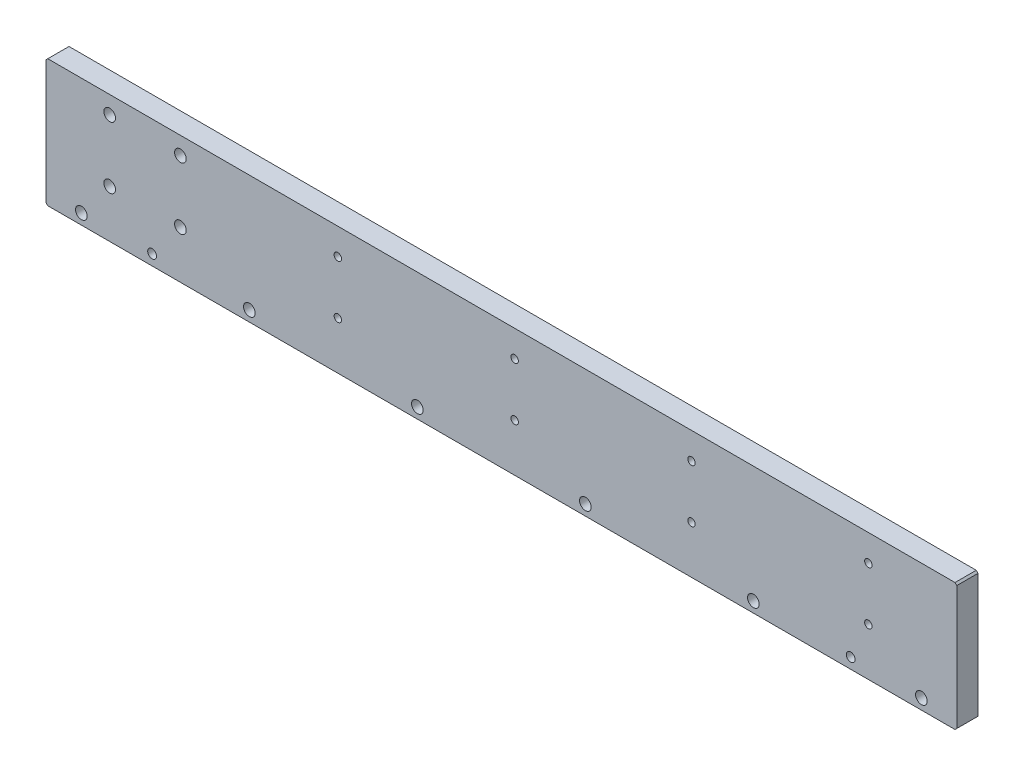
from build123d import *

# Parameters (mm, degrees)
SKETCH1_W                                           = 515
SKETCH1_H                                           = 72
BOSS_EXTRUDE1_DEPTH                                 = 6
M5_TAPPED_HOLE1_D                                   = 4.2
BLIND_PIN_HOLE0_D                                   = 5
BLIND_PIN_HOLE0_DEPTH                               = 10
BLIND_PIN_HOLE0_TIP                                 = 1.502151548
CBORE_FOR_M6_HEX_SOCKET_HEAD_CAP_SCREW1_D           = 6.6
CBORE_FOR_M6_HEX_SOCKET_HEAD_CAP_SCREW1_CBORE_D     = 11
CBORE_FOR_M6_HEX_SOCKET_HEAD_CAP_SCREW1_CBORE_DEPTH = 6.4
BLIND_PIN_HOLE1_D                                   = 5
BLIND_PIN_HOLE1_DEPTH                               = 10
BLIND_PIN_HOLE1_TIP                                 = 1.502151548
CBORE_FOR_M6_HEX_SOCKET_HEAD_CAP_SCREW2_D           = 6.6
CBORE_FOR_M6_HEX_SOCKET_HEAD_CAP_SCREW2_CBORE_D     = 11
CBORE_FOR_M6_HEX_SOCKET_HEAD_CAP_SCREW2_CBORE_DEPTH = 6.4
CHAMFER1_SIZE                                       = 1


with BuildPart() as part:
    # Sketch1 → Boss-Extrude1 (new, symmetric)
    with BuildSketch(Plane.XY):
        Rectangle(SKETCH1_W, SKETCH1_H)
    extrude(amount=BOSS_EXTRUDE1_DEPTH, both=True)

    # M5 Tapped Hole1 (through all)
    with Locations(Plane.XY.offset(6)):
        with Locations((207.5, -9), (207.5, 21), (107.5, -9), (107.5, 21), (7.5, -9), (7.5, 21), (-92.5, -9), (-92.5, 21)):
            Hole(M5_TAPPED_HOLE1_D / 2)

    # Blind pin hole0
    with Locations(Plane(origin=(0, 0, -6), x_dir=(1, 0, 0), z_dir=(0, 0, -1))):
        with Locations((227.5, 26.5), (-122.5, 26.5)):
            Hole(BLIND_PIN_HOLE0_D / 2, depth=BLIND_PIN_HOLE0_DEPTH)
            with Locations((0, 0, -(BLIND_PIN_HOLE0_DEPTH + BLIND_PIN_HOLE0_TIP / 2))):  # 118° drill point
                Cone(0, BLIND_PIN_HOLE0_D / 2, BLIND_PIN_HOLE0_TIP, mode=Mode.SUBTRACT)

    # CBORE for M6 Hex Socket Head Cap Screw1 (through all)
    with Locations(Plane(origin=(0, 0, -6), x_dir=(1, 0, 0), z_dir=(0, 0, -1))):
        with Locations((-237.5, 30), (-142.5, 30), (-47.5, 30), (47.5, 30), (142.5, 30), (237.5, 30)):
            CounterBoreHole(CBORE_FOR_M6_HEX_SOCKET_HEAD_CAP_SCREW1_D / 2, CBORE_FOR_M6_HEX_SOCKET_HEAD_CAP_SCREW1_CBORE_D / 2, CBORE_FOR_M6_HEX_SOCKET_HEAD_CAP_SCREW1_CBORE_DEPTH)

    # Blind pin hole1
    with Locations(Plane.XY.offset(6)):
        with Locations((-197.5, -30), (197.5, -30)):
            Hole(BLIND_PIN_HOLE1_D / 2, depth=BLIND_PIN_HOLE1_DEPTH)
            with Locations((0, 0, -(BLIND_PIN_HOLE1_DEPTH + BLIND_PIN_HOLE1_TIP / 2))):  # 118° drill point
                Cone(0, BLIND_PIN_HOLE1_D / 2, BLIND_PIN_HOLE1_TIP, mode=Mode.SUBTRACT)

    # CBORE for M6 Hex Socket Head Cap Screw2 (through all)
    with Locations(Plane(origin=(0, 0, -6), x_dir=(-1, 0, 0), z_dir=(0, 0, -1))):
        with Locations((181.5, 26), (221.5, -9), (181.5, -9), (221.5, 26)):
            CounterBoreHole(CBORE_FOR_M6_HEX_SOCKET_HEAD_CAP_SCREW2_D / 2, CBORE_FOR_M6_HEX_SOCKET_HEAD_CAP_SCREW2_CBORE_D / 2, CBORE_FOR_M6_HEX_SOCKET_HEAD_CAP_SCREW2_CBORE_DEPTH)

    # Chamfer1
    chamfer1_edges = [part.edges().sort_by_distance(p)[0] for p in [
        (257.5, -36, 0),
        (-257.5, -36, 0),
        (-257.5, 36, 0),
        (257.5, 36, 0),
    ]]
    chamfer(chamfer1_edges, length=CHAMFER1_SIZE)


solid = part.part
